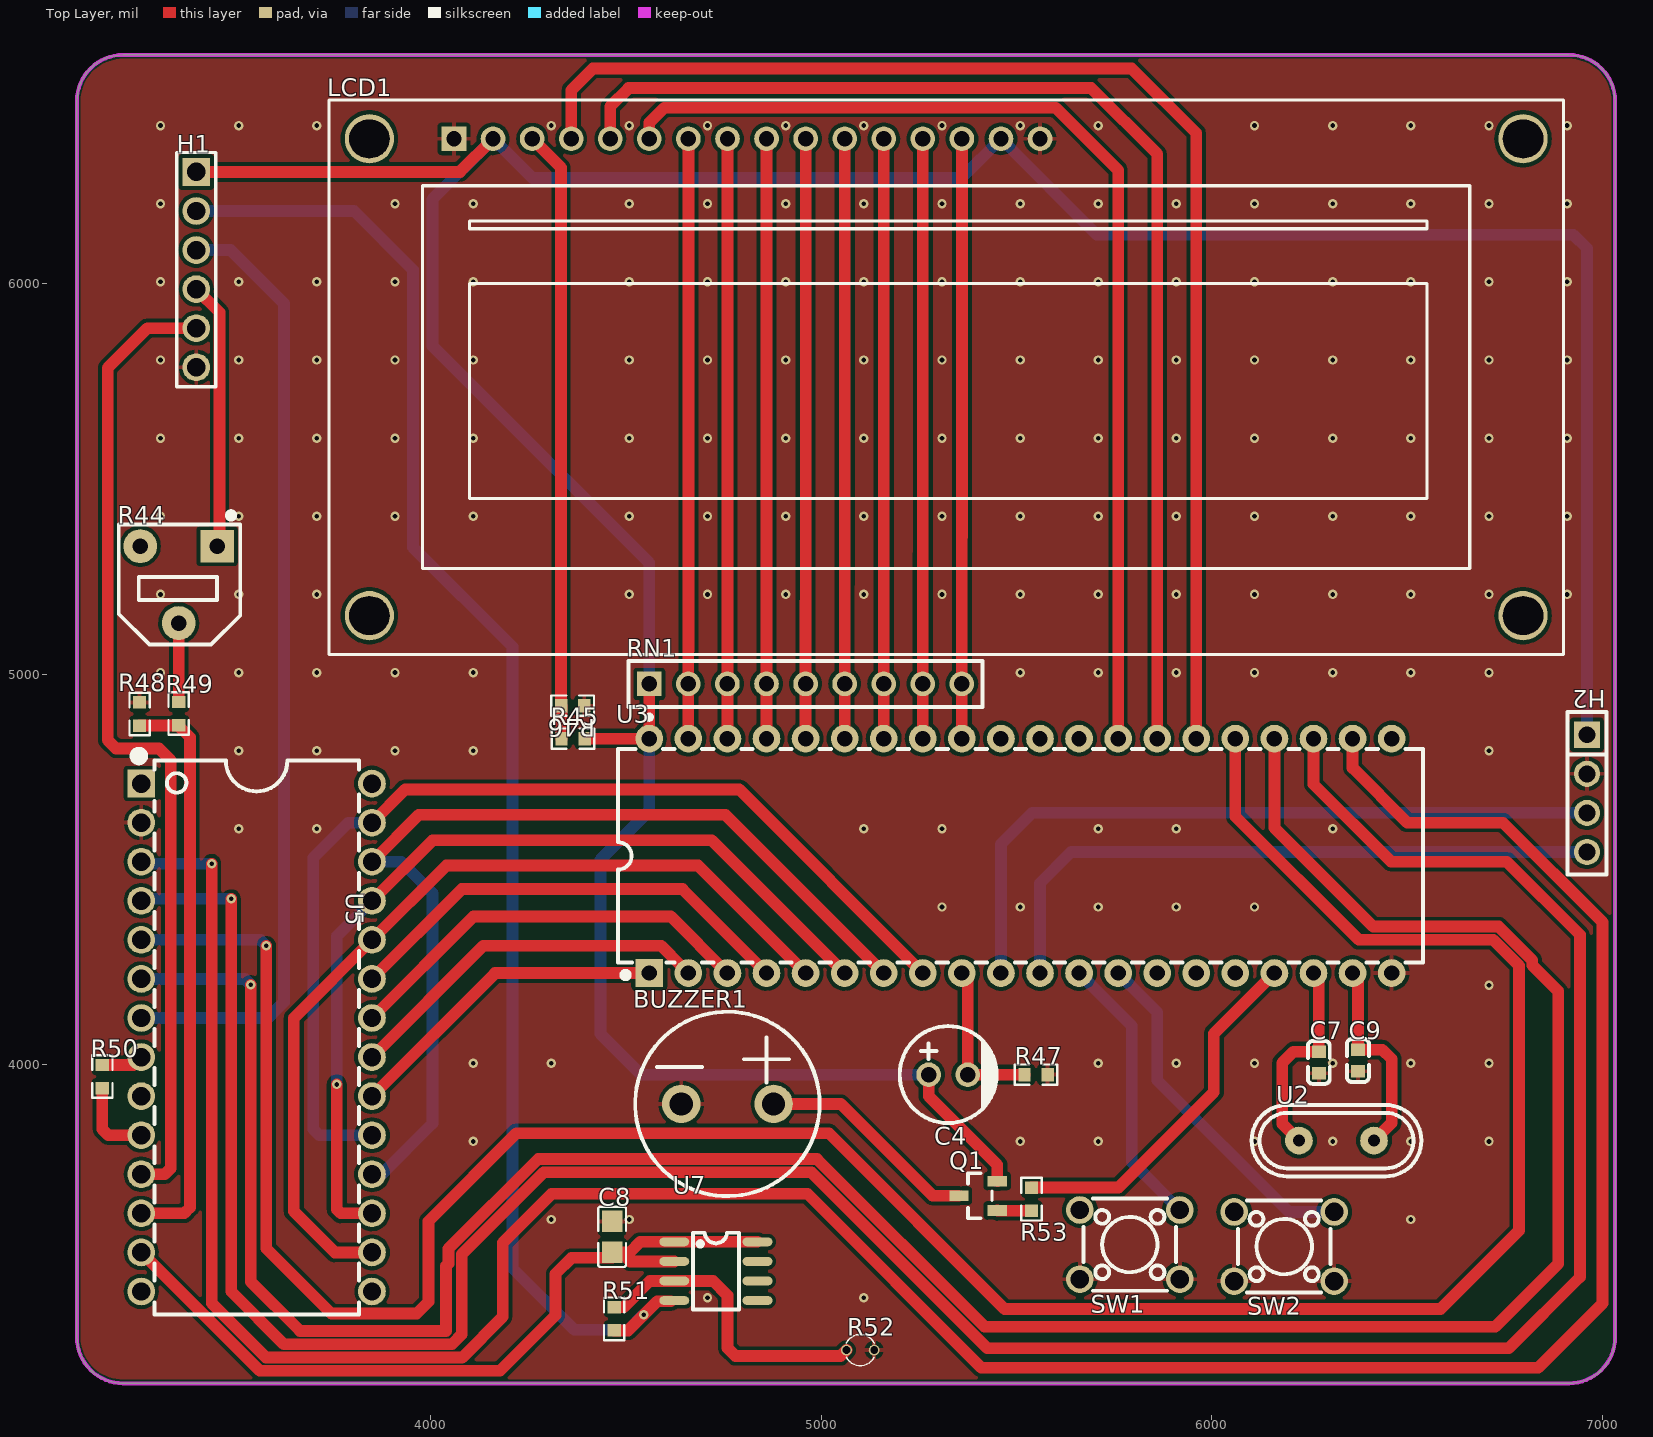
[diagram p0: Top Layer view]
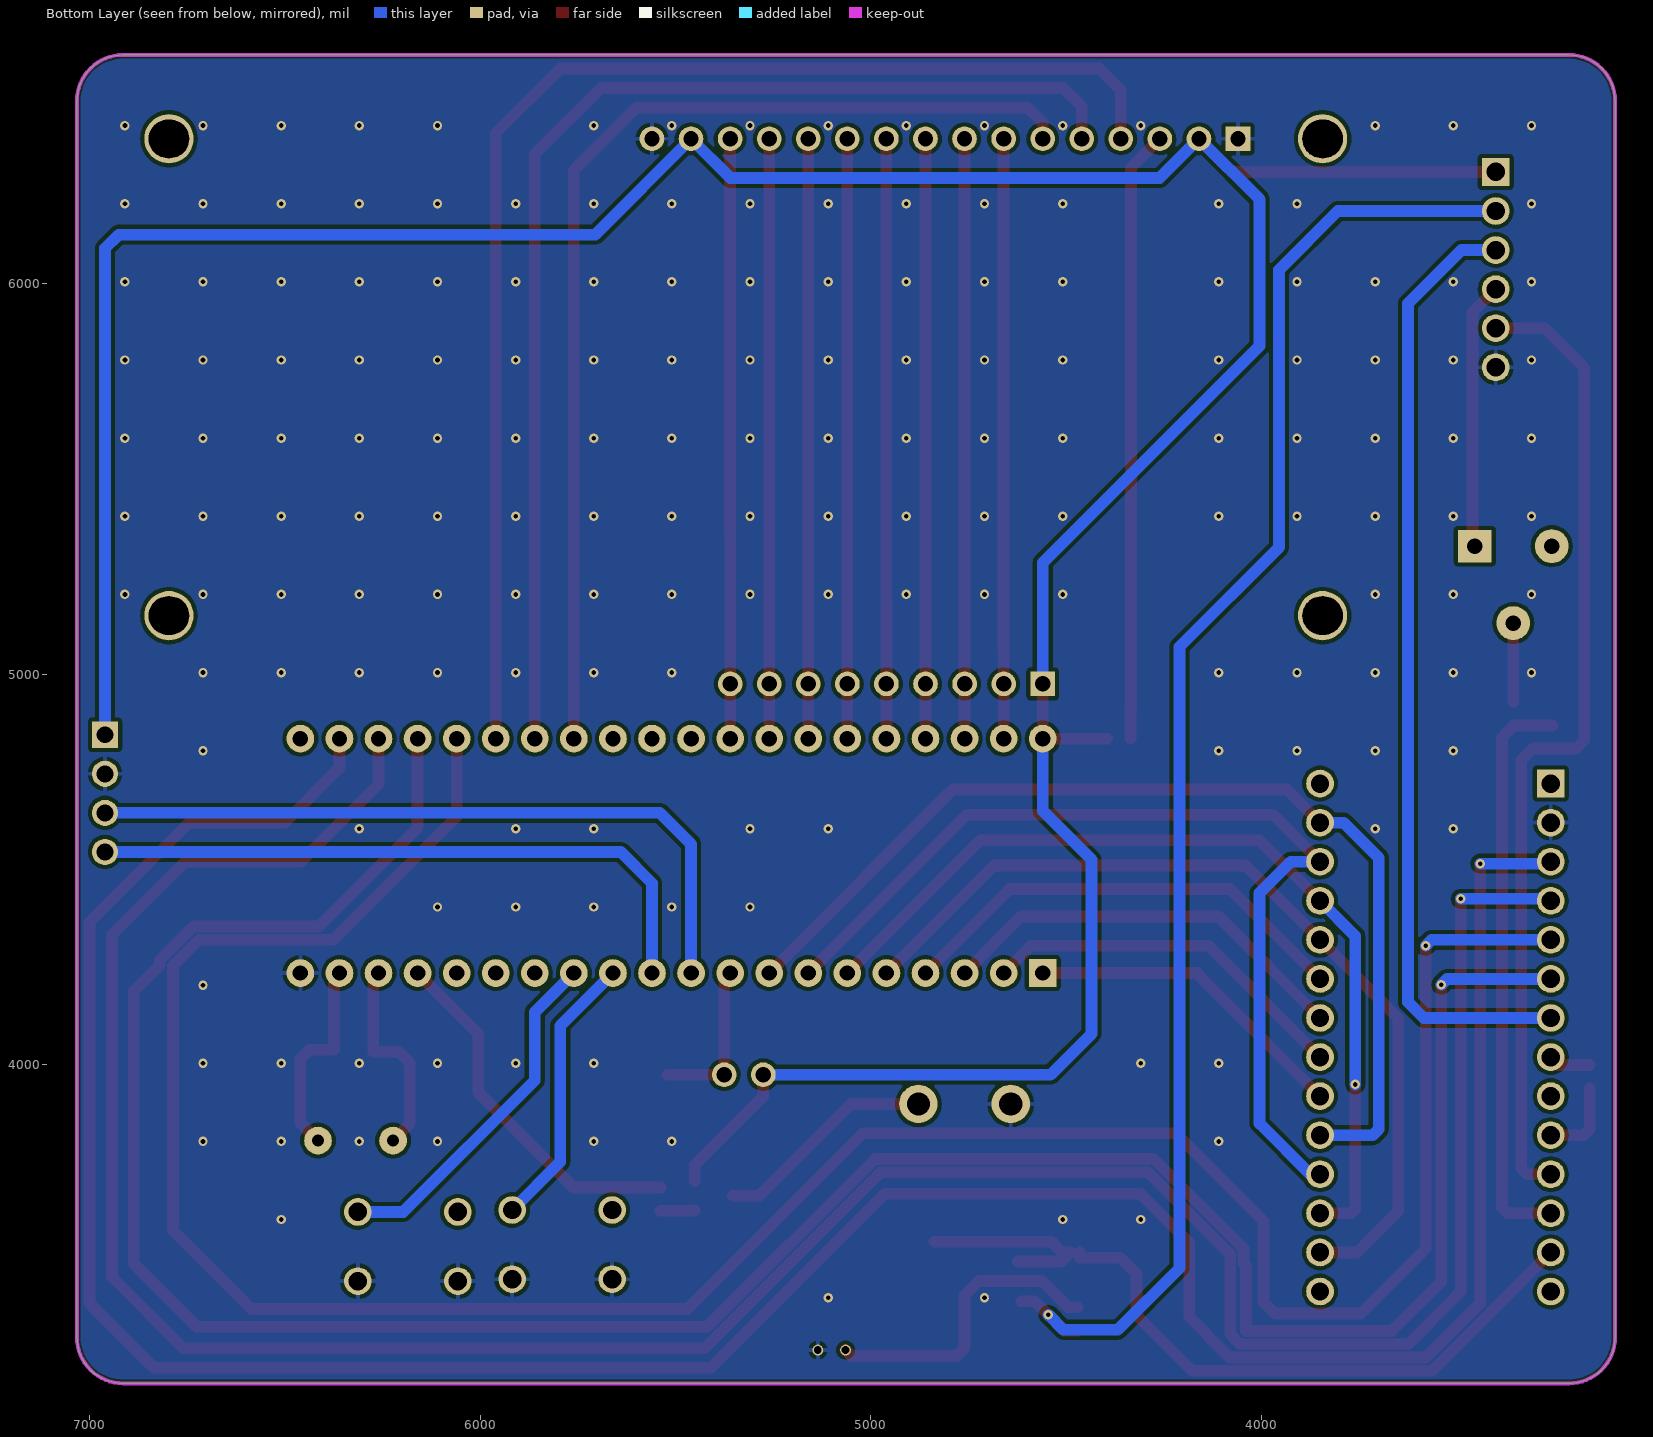
[diagram p1: Bottom Layer view, seen from below]
# Altium PCB MISC51839.pcbdoc
Units mil, origin at the board's own origin, x right, y up, seen from the top; angles counter-clockwise.
Board outline 3937.01 x 3400.14 mil, 2 copper layers (Top Layer, Bottom Layer), stack 62.206 mil thick; 26 components, 49 nets, 159 pads, 176 vias.

## Layer stack, top to bottom
Top Solder Mask Layer: solder mask 0.394, Dk 3.3
Top Layer: signal copper 1.379
Dielectric1: surface 59.449, FR4, Dk 4.5
Bottom Layer: signal copper 1.378
Bottom Solder Mask Layer: solder mask 0.394, Dk 3.3

## Board outline
3213.11,6585 ccw(c3213.11,6466.89) 3095,6466.89 3095,3302.97 ccw(c3213.11,3302.97) 3213.11,3184.86 6913.9,3184.86 ccw(c6913.9,3302.97) 7032.01,3302.97 7032.01,6466.89 ccw(c6913.9,6466.89) 6913.9,6585

## Design rules (kind name [scope] priority, off if disabled: settings)
BoardOutlineClearance copperThickness2oz_1 [All] p2 off: genericclearance=7.99 ignorepadtopadclearanceinfootprint=FALSE except(0: Arc-SplitContinuation Track-SplitContinuation SMDPad-SplitContinuation THPad-SplitContinuation Via-SplitContinuation Fill-SplitContinuation Region-SplitContinuation Poly-SplitContinuation Text-SplitContinuation Hole-SplitContinuation; 5.98: Arc-CutoutEdge Track-CutoutEdge SMDPad-CutoutEdge THPad-CutoutEdge Via-CutoutEdge Text-CutoutEdge; 6.9: Hole-OutlineEdge Hole-CutoutEdge; 10: Poly-OutlineEdge Poly-CutoutEdge; 11.81: Arc-OutlineEdge Track-OutlineEdge SMDPad-OutlineEdge THPad-OutlineEdge Via-OutlineEdge Fill-OutlineEdge Region-OutlineEdge Text-OutlineEdge Fill-CutoutEdge Region-CutoutEdge)
BoardOutlineClearance Plane_innerPlane_1 [All] p4 off: genericclearance=4.02 ignorepadtopadclearanceinfootprint=FALSE except(0: Arc-SplitContinuation Track-SplitContinuation SMDPad-SplitContinuation THPad-SplitContinuation Via-SplitContinuation Fill-SplitContinuation Region-SplitContinuation Poly-SplitContinuation Text-SplitContinuation Hole-SplitContinuation; 5.98: Arc-CutoutEdge Track-CutoutEdge SMDPad-CutoutEdge THPad-CutoutEdge Via-CutoutEdge Text-CutoutEdge; 6.9: Hole-OutlineEdge Hole-CutoutEdge; 10: Poly-OutlineEdge Poly-CutoutEdge; 11.81: Arc-OutlineEdge Track-OutlineEdge SMDPad-OutlineEdge THPad-OutlineEdge Via-OutlineEdge Fill-OutlineEdge Region-OutlineEdge Text-OutlineEdge Fill-CutoutEdge Region-CutoutEdge)
BoardOutlineClearance Copper_copperRegion_1 [All] p6 off: genericclearance=4.02 ignorepadtopadclearanceinfootprint=FALSE except(0: Arc-SplitContinuation Track-SplitContinuation SMDPad-SplitContinuation THPad-SplitContinuation Via-SplitContinuation Fill-SplitContinuation Region-SplitContinuation Poly-SplitContinuation Text-SplitContinuation Hole-SplitContinuation; 5.98: Arc-CutoutEdge Track-CutoutEdge SMDPad-CutoutEdge THPad-CutoutEdge Via-CutoutEdge Text-CutoutEdge; 6.9: Hole-OutlineEdge Hole-CutoutEdge; 10: Poly-OutlineEdge Poly-CutoutEdge; 11.81: Arc-OutlineEdge Track-OutlineEdge SMDPad-OutlineEdge THPad-OutlineEdge Via-OutlineEdge Fill-OutlineEdge Region-OutlineEdge Text-OutlineEdge Fill-CutoutEdge Region-CutoutEdge)
BoardOutlineClearance copperThickness1oz_1 [All] p8: genericclearance=4.02 ignorepadtopadclearanceinfootprint=FALSE except(0: Arc-SplitContinuation Track-SplitContinuation SMDPad-SplitContinuation THPad-SplitContinuation Via-SplitContinuation Fill-SplitContinuation Region-SplitContinuation Poly-SplitContinuation Text-SplitContinuation Hole-SplitContinuation; 5.98: Arc-CutoutEdge Track-CutoutEdge SMDPad-CutoutEdge THPad-CutoutEdge Via-CutoutEdge Text-CutoutEdge; 6.9: Hole-OutlineEdge Hole-CutoutEdge; 10: Poly-OutlineEdge Poly-CutoutEdge; 11.81: Arc-OutlineEdge Track-OutlineEdge SMDPad-OutlineEdge THPad-OutlineEdge Via-OutlineEdge Fill-OutlineEdge Region-OutlineEdge Text-OutlineEdge Fill-CutoutEdge Region-CutoutEdge)
Clearance copperThickness2oz [All] p1 off: gap=7.99 ignorepadtopadclearanceinfootprint=FALSE except(5.98: SMDPad-Track SMDPad-SMDPad THPad-Track SMDPad-THPad THPad-THPad Track-Via SMDPad-Via THPad-Via Via-Via Fill-SMDPad Region-SMDPad Fill-THPad Region-THPad Fill-Via Region-Via Fill-Fill Fill-Region Region-Region Arc-Track Arc-SMDPad Arc-THPad Arc-Via Fill-Arc Region-Arc Arc-Arc Text-Track SMDPad-Text Text-THPad Text-Via Fill-Text Region-Text Arc-Text Text-Text; 6.9: Hole-Track Hole-SMDPad Hole-THPad Hole-Via Fill-Hole Region-Hole Hole-Arc Hole-Text; 10: Poly-Track Poly-SMDPad Poly-THPad Poly-Via Poly-Fill Poly-Region Poly-Poly Poly-Arc Poly-Text Poly-Hole; 11.81: Fill-Track Region-Track)
Clearance Plane_innerPlane [All] p3 off: gap=4.02 ignorepadtopadclearanceinfootprint=FALSE except(5.98: SMDPad-Track SMDPad-SMDPad THPad-Track SMDPad-THPad THPad-THPad Track-Via SMDPad-Via THPad-Via Via-Via Fill-SMDPad Region-SMDPad Fill-THPad Region-THPad Fill-Via Region-Via Fill-Fill Fill-Region Region-Region Arc-Track Arc-SMDPad Arc-THPad Arc-Via Fill-Arc Region-Arc Arc-Arc Text-Track SMDPad-Text Text-THPad Text-Via Fill-Text Region-Text Arc-Text Text-Text; 6.9: Hole-Track Hole-SMDPad Hole-THPad Hole-Via Fill-Hole Region-Hole Hole-Arc Hole-Text; 10: Poly-Track Poly-SMDPad Poly-THPad Poly-Via Poly-Fill Poly-Region Poly-Poly Poly-Arc Poly-Text Poly-Hole; 11.81: Fill-Track Region-Track)
Clearance Copper_copperRegion [All] p5 off: gap=4.02 ignorepadtopadclearanceinfootprint=FALSE except(5.98: SMDPad-Track SMDPad-SMDPad THPad-Track SMDPad-THPad THPad-THPad Track-Via SMDPad-Via THPad-Via Via-Via Fill-SMDPad Region-SMDPad Fill-THPad Region-THPad Fill-Via Region-Via Fill-Fill Fill-Region Region-Region Arc-Track Arc-SMDPad Arc-THPad Arc-Via Fill-Arc Region-Arc Arc-Arc Text-Track SMDPad-Text Text-THPad Text-Via Fill-Text Region-Text Arc-Text Text-Text; 6.9: Hole-Track Hole-SMDPad Hole-THPad Hole-Via Fill-Hole Region-Hole Hole-Arc Hole-Text; 10: Poly-Track Poly-SMDPad Poly-THPad Poly-Via Poly-Fill Poly-Region Poly-Poly Poly-Arc Poly-Text Poly-Hole; 11.81: Fill-Track Region-Track)
Clearance copperThickness1oz [All] p7: gap=4.02 ignorepadtopadclearanceinfootprint=FALSE except(5.98: SMDPad-Track SMDPad-SMDPad THPad-Track SMDPad-THPad THPad-THPad Track-Via SMDPad-Via THPad-Via Via-Via Fill-SMDPad Region-SMDPad Fill-THPad Region-THPad Fill-Via Region-Via Fill-Fill Fill-Region Region-Region Arc-Track Arc-SMDPad Arc-THPad Arc-Via Fill-Arc Region-Arc Arc-Arc Text-Track SMDPad-Text Text-THPad Text-Via Fill-Text Region-Text Arc-Text Text-Text; 6.9: Hole-Track Hole-SMDPad Hole-THPad Hole-Via Fill-Hole Region-Hole Hole-Arc Hole-Text; 10: Poly-Track Poly-SMDPad Poly-THPad Poly-Via Poly-Fill Poly-Region Poly-Poly Poly-Arc Poly-Text Poly-Hole; 11.81: Fill-Track Region-Track)
DiffPairsRouting differentialPair [All] p1: maxlimit=6 minlimit=6 mostfreqgap=6 toplayer_minwidth=5 toplayer_prefwidth=10 toplayer_maxwidth=100 toplayer_mingap=6 toplayer_prefgap=6 toplayer_maxgap=6 bottomlayer_minwidth=5 bottomlayer_prefwidth=10 bottomlayer_maxwidth=100 bottomlayer_mingap=6 bottomlayer_prefgap=6 bottomlayer_maxgap=6 maxuncoupledlength=10
HoleToHoleClearance otherClearance [All] p1: gap=11.81 allowstackedmicrovias=TRUE
Length netLength [All] p1: minlimit=0 maxlimit=0
PasteMaskExpansion pasteMaskExpansion [All] p1: expansion=0
PlaneConnect innerPlane [All] p1: planeconnectstyle=Relief reliefexpansion=20 reliefentries=4 reliefconductorwidth=10 reliefairgap=10
PolygonConnect copperRegion [All] p1: connectstyle=Relief reliefconductorwidth=10 reliefentries=4 polygonreliefangle="90 Angle" airgapwidth=10 via.connectstyle=Relief via.reliefconductorwidth=10 via.reliefentries=4 via.polygonreliefangle="90 Angle" via.airgapwidth=10
RoutingVias viaSize [All] p1: holewidth=12.01 width=24.02 viastyle="Through Hole" minholewidth=11.81 minwidth=19.68 maxholewidth=248.03 maxwidth=393.7
SolderMaskExpansion solderMaskExpansion [IsVia] p1: expansion=-1000 istentingtop=TRUE
SolderMaskExpansion solderMaskExpansion [All] p2: expansion=2 istentingtop=FALSE
Width copperThickness2oz_2 [All] p1 off: maxlimit=100 minlimit=8 preferedwidth=10
Width copperThickness1oz_2 [All] p2: maxlimit=100 minlimit=5 preferedwidth=10

## Components (designator, comment, footprint, x,y, rotation, side; value= is the part's Value field where it differs from the comment)
BUZZER1 "buzzer" BUZ-TH_BD12.0-P6.00-D0.9-RD 4760,3900 r0 top
C4 "10uF" CAP-TH_BD6.3-P2.50-D1.0-FD 5325,3975 r0 top
C7 "22pF" C0603 6273.79,4006.21 r90 top
C8 "100nF" C0805 4465,3560 r270 top
C9 "22pF" C0603 6373.79,4011.21 r90 top
H1 "" HDR-TH_6P-P2.54-V-M-1 3400.49,6035.49 r270 top
H2 "" HDR-TH_4P-P2.54-V-F 6960,4695 r270 top
LCD1 "LMB162ADC" LCD1602 5320,5760 r0 top
Q1 "" S8550P_SOT 5400,3665 r0 top
R44 "10kΩ" RES-ADJ-SMD_RM065-V1 3355.64,5229.2 r180 top
R45 "10K" R0603 4365,4835 r0 top
R46 "1K" R0603 4363.85,4919.21 r180 top
R47 "10K" R0603 5550,3975 r180 top
R48 "100K" R0603 3255.5,4898.03 r90 top
R49 "100K" R0603 3355.64,4899.2 r90 top
R50 "50" R0603 3160,3970 r90 top
R51 "1K" R0603 4470,3350 r270 top
R52 "MF52A502F3435" RES-TH_BD2.0-P1.80-D0.3 5100,3270 r180 top
R53 "2.2K" R0603 5538.43,3656.2 r270 top
RN1 "-" RES-ARRAY-TH_9P-P2.54-D1.0 4960,4975 r0 top
SW1 "" SW-TH_4P-L6.0-W6.0-P4.50-LS6.5 5790,3540 r180 top
SW2 "" SW-TH_4P-L6.0-W6.0-P4.50-LS6.5 6185,3535 r180 top
U2 "12MHz" HC-49US_L11.0-W4.6-P4.88 6318.79,3806.21 r0 top
U3 "STC89C516RD+40I-PDIP40" DIP-40_L52.3-W13.9-P2.54-LS15.2-BL 5510,4535 r0 top
U5 "AD1674AD" CDIP-28_L35.5-W14.8-P2.54-LS15.3-BL 3555,4070 r270 top
U7 "LM358P-CN" SOIC-8_L5.0-W4.0-P1.27-LS6.0-BL 4730.48,3471.93 r270 top

## Footprints (in the part's own frame and the unit in brackets; to place one, negate y for a bottom-side part, rotate by r counter-clockwise, add the part's x,y. Pads: shape width x height; smd on the part's side, far side on the other; paste and mask are expansions set on the pad)
BUZ-TH_BD12.0-P6.00-D0.9-RD [mm]
  round 2.5 hole 1.5 paste+0 mask+0.05: 1(-3,0) 2(3,0)
  silkscreen extent -5.99,-5.99 5.99,5.99
C0603 [mm]
  rect 0.8x0.9 smd: 1(-0.7,0) 2(0.7,0)
  silkscreen extent -1.39,-0.71 1.39,0.71
C0805 [mm]
  rect 1.41x1.35 smd paste-100 mask+0.051: 1(-1,0) 2(1,0)
  silkscreen extent -1.96,-0.9 1.96,0.9
CAP-TH_BD6.3-P2.50-D1.0-FD [mm]
  round 1.6 hole 1: 1(-1.27,0) 2(1.27,0)
  silkscreen extent -3.15,-3.15 3.17,3.15
CDIP-28_L35.5-W14.8-P2.54-LS15.3-BL [mm]
  rect 1.8x1.8 hole 1.2: 1(-16.51,-7.5)
  round 1.8 hole 1.2: 2(-13.97,-7.5) 3(-11.43,-7.5) 4(-8.89,-7.5) 5(-6.35,-7.5) 6(-3.81,-7.5) 7(-1.27,-7.5) 8(1.27,-7.5) 9(3.81,-7.5) 10(6.35,-7.5) 11(8.89,-7.5) 12(11.43,-7.5) 13(13.97,-7.5) 14(16.51,-7.5) 15(16.51,7.5) 16(13.97,7.5) 17(11.43,7.5) 18(8.89,7.5) 19(6.35,7.5) 20(3.81,7.5) 21(1.27,7.5) 22(-1.27,7.5) 23(-3.81,7.5) 24(-6.35,7.5) 25(-8.89,7.5) 26(-11.43,7.5) 27(-13.97,7.5) 28(-16.51,7.5)
  silkscreen extent -18.6,-7.96 18,6.65
DIP-40_L52.3-W13.9-P2.54-LS15.2-BL [mm]
  rect 1.8x1.8 hole 1: 1(-24.13,-7.62)
  round 1.8 hole 1: 2(-21.59,-7.62) 3(-19.05,-7.62) 4(-16.51,-7.62) 5(-13.97,-7.62) 6(-11.43,-7.62) 7(-8.89,-7.62) 8(-6.35,-7.62) 9(-3.81,-7.62) 10(-1.27,-7.62) 11(1.27,-7.62) 12(3.81,-7.62) 13(6.35,-7.62) 14(8.89,-7.62) 15(11.43,-7.62) 16(13.97,-7.62) 17(16.51,-7.62) 18(19.05,-7.62) 19(21.59,-7.62) 20(24.13,-7.62) 21(24.13,7.62) 22(21.59,7.62) 23(19.05,7.62) 24(16.51,7.62) 25(13.97,7.62) 26(11.43,7.62) 27(8.89,7.62) 28(6.35,7.62) 29(3.81,7.62) 30(1.27,7.62) 31(-1.27,7.62) 32(-3.81,7.62) 33(-6.35,7.62) 34(-8.89,7.62) 35(-11.43,7.62) 36(-13.97,7.62) 37(-16.51,7.62) 38(-19.05,7.62) 39(-21.59,7.62) 40(-24.13,7.62)
  silkscreen extent -26.16,-7.95 26.16,6.93
HC-49US_L11.0-W4.6-P4.88 [mm]
  round 1.8 hole 0.8: 1(-2.44,0) 2(2.44,0)
  silkscreen extent -5.51,-2.32 5.51,2.32
HDR-TH_4P-P2.54-V-F [mm]
  rect 1.7x1.7 hole 1.1: 1(-3.81,0)
  round 1.7 hole 1.1: 2(-1.27,0) 3(1.27,0) 4(3.81,0)
  silkscreen extent -5.29,-1.27 5.29,1.27
HDR-TH_6P-P2.54-V-M-1 [mm]
  rect 1.8x1.8 hole 1.2: 1(-6.35,0)
  round 1.8 hole 1.2: 2(-3.81,0) 3(-1.27,0) 4(1.27,0) 5(3.81,0) 6(6.35,0)
  silkscreen extent -7.62,-1.27 7.62,1.27
LCD1602 [mm]
  round 3.2 hole 2.5 slot 2.625 at 0 deg: 0(-37.5,-15.5) 0(-37.5,15.5) 0(37.5,-15.5) 0(37.5,15.5)
  rect 1.6x1.6 hole 1: 1(-32,15.5)
  round 1.6 hole 1: 2(-29.46,15.5) 3(-26.92,15.5) 4(-24.38,15.5) 5(-21.84,15.5) 6(-19.3,15.5) 7(-16.76,15.5) 8(-14.22,15.5) 9(-11.68,15.5) 10(-9.14,15.5) 11(-6.6,15.5) 12(-4.06,15.5) 13(-1.52,15.5) 14(1.02,15.5) 15(3.56,15.5) 16(6.1,15.5)
  silkscreen extent -40.13,-18.03 40.13,18.03
R0603 [mil]
  rect 31.75x34.02 smd paste-3937.01 mask+2: 1(-29.66,0) 2(29.66,0)
  silkscreen extent -55,-26 55,26
RES-ADJ-SMD_RM065-V1 [mm]
  rect 2.2x2.1 hole 1 paste+0 mask+0.05: 1(-2.5,-2.5)
  round 2.2 hole 1 paste+0 mask+0.05: 2(0,2.5) 3(2.5,-2.5)
  silkscreen extent -4,-4.7 3.9,3.9
RES-ARRAY-TH_9P-P2.54-D1.0 [mm]
  rect 1.6x1.6 hole 1: 1(-10.16,0)
  round 1.6 hole 1: 2(-7.62,0) 3(-5.08,0) 4(-2.54,0) 5(0,0) 6(2.54,0) 7(5.08,0) 8(7.62,0) 9(10.16,0)
  silkscreen extent -11.5,-2.31 11.5,1.5
RES-TH_BD2.0-P1.80-D0.3 [mm]
  round 0.7 hole 0.5 paste+0 mask+0.05: 1(-0.9,0) 2(0.9,0)
  silkscreen extent -0.91,-1.01 0.91,1.01
S8550P_SOT [mil]
  rect 49.2x27.6 smd paste+0 mask+2: 1(50.84,-37.4) 2(50.84,37.4) 3(-47.56,0)
  silkscreen extent -24,-58 37,58
SOIC-8_L5.0-W4.0-P1.27-LS6.0-BL [mil]
  oval 22.38x76.78 smd: 1(-75,-106.5) 2(-25,-106.5) 3(25,-106.5) 4(75,-106.5) 5(75,106.5) 6(25,106.5) 7(-25,106.5) 8(-75,106.5)
  silkscreen extent -98,-59 98,59
SW-TH_4P-L6.0-W6.0-P4.50-LS6.5 [mm]
  round 1.8 hole 1.2: 1(-3.25,2.25) 2(3.25,2.25) 3(-3.25,-2.25) 4(3.25,-2.25)
  silkscreen extent -3,-3 3,3

## Via types
v1: diameter 24.02, hole 12, Top Layer to Bottom Layer, 176 vias

## Nets (pads, with @x,y where several pads share a name; then routed paths per layer and width w, separated by ;. In a path a pad name is that pad's centre, name@x,y a point inside that pad or via, vN(x,y) a via of type N, cw(c..) or ccw(c..) an arc to the next point about the centre after c; other vN are vias at no path point)
$1N1586: LCD1.14 RN1.9 U3.32 | length 1535.3
  Top Layer w30: U3.32 RN1.9 5360,5351.13 5360.16,5351.29 LCD1.14
$1N1590: LCD1.7 RN1.2 U3.39 | length 1535.3
  Top Layer w30: U3.39 RN1.2 4660,5061.18 4660.16,5061.34 LCD1.7
$1N1591: LCD1.8 RN1.3 U3.38 | length 1535.3
  Top Layer w30: U3.38 RN1.3 4760,5102.6 4760.16,5102.76 LCD1.8
$1N1592: LCD1.9 RN1.4 U3.37 | length 1535.3
  Top Layer w30: U3.37 RN1.4 4860,5144.02 4860.16,5144.18 LCD1.9
$1N1593: LCD1.10 RN1.5 U3.36 | length 1535.3
  Top Layer w30: U3.36 RN1.5 4960,5185.44 4960.16,5185.6 LCD1.10
$1N1594: LCD1.11 RN1.6 U3.35 | length 1535.3
  Top Layer w30: U3.35 RN1.6 5060,5226.86 5060.16,5227.02 LCD1.11
$1N1595: LCD1.12 RN1.7 U3.34 | length 1535.3
  Top Layer w30: U3.34 RN1.7 5160,5268.28 5160.16,5268.44 LCD1.12
$1N1596: LCD1.13 RN1.8 U3.33 | length 1535.3
  Top Layer w30: U3.33 RN1.8 5260,5309.7 5260.16,5309.86 LCD1.13
$1N1605: LCD1.3 R45.1 R46.2 | length 1566.4
  Top Layer w30: LCD1.3 4334.19,6296.21 R46.2 4335.34,4918.06 R45.1
$1N1611: C7.2 U2.1 U3.18 | length 529.1
  Top Layer w30: U2.1 6180,3848.94 6180,4005 6208.77,4033.77 C7.2 6273.79,4221.21 U3.18
$1N1612: C9.2 U2.2 U3.19 | length 525.5
  Top Layer w30: U3.19 6373.79,4221.21 C9.2 6436.23,4038.77 6460,4015 6460,3851.36 U2.2@6414.85,3806.21
$1N22801: C4.2 R47.2 U3.9 | length 411.6
  Top Layer w30: U3.9 5375,4220 C4.2 R47.2
$1N22819: U3.1 U5.20 | length 840.2
  Top Layer w30: U5.20 4165.27,4235 U3.1
$1N22823: U3.2 U5.21 | length 957.1
  Top Layer w30: U5.21 4135.27,4305 4590.54,4305 4616.42,4279.12 4616.42,4278.58 U3.2
$1N22827: U3.8 U5.19 U5.27 | length 2678.6
  Top Layer w30: U5.27 3935.27,4705 4790,4705 U3.8
  Bottom Layer w30: U5.19 3715,3820 3700,3835 3700,4530 3790,4620 U5.27
$1N22836: U3.7 U5.18 U5.26 | length 2513.6
  Top Layer w30: U5.26 3970.27,4640 4755,4640 U3.7
  Bottom Layer w30: U5.18 3875,3720 4005,3850 4005,4440 3925,4520 U5.26
$1N22841: U3.6 U5.17 U5.25 | length 2336.6
  Top Layer w30: v1(3760,3950) 3760,3630 3770,3620 U5.17 ; U5.25 4005.27,4575 4720,4575 U3.6
  Bottom Layer w30: v1(3760,3950) 3760,4329.73 U5.25
$1N22846: U3.5 U5.16 U5.24 | length 2324.1
  Top Layer w30: U5.16 3755,3520 3650,3625 3650,4119.73 U5.24 4040.27,4510 4685,4510 U3.5
$1N22851: U3.4 U5.23 | length 1194.1
  Top Layer w30: U5.23 4080.27,4450 4645,4450 U3.4
$1N22856: U3.3 U5.22 | length 1077.5
  Top Layer w30: U5.22 4110.27,4380 4615,4380 U3.3
$1N23012: R50.2 U5.8 | length 108.2
  Top Layer w30: R50.2 3239.39,3999.66 U5.8
$1N23018: R50.1 U5.10 | length 211.3
  Top Layer w30: R50.1 3160,3835 3175,3820 U5.10
$1N23025: R48.1 R49.1 U5.12 | length 1477.4
  Top Layer w30: R48.1 R49.1@3354.47,4868.37 ; U5.12 3369.47,3620 3384.47,3635 3384.47,4838.37 R49.1@3354.47,4868.37 ; R49.1 R49.1@3354.47,4868.37
$1N23497: C8.2 U5.13 U7.1 U7.2 U7.8 | length 2033.2
  Top Layer w30: U5.13 3562.92,3216.81 4178,3216.81 4320,3358.81 4320,3465 4361.08,3506.08 4465,3506.08 C8.2 ; U7.2 4511.64,3496.93 4487.95,3520.63 4510.63,3520.63 4536.93,3546.93 U7.1 U7.8
$1N23895: R51.1 R52.2 U7.3 | length 786.9
  Top Layer w30: R51.1 4494.66,3379.66 4561.93,3446.93 U7.3 4723.07,3446.93 4760,3410 4760,3275.52 4780.52,3255 5049.56,3255 R52.2
$1N24757: R44.2 R49.2 | length 201.9
  Top Layer w30: R49.2 R44.2
$1N26077: H2.3 U3.10 | length 1863.1
  Bottom Layer w30: U3.10 5460,4565 5540,4645 H2.3
$1N26083: H2.4 U3.11 | length 1663.1
  Bottom Layer w30: U3.11 5560,4465 5640,4545 H2.4
$1N26653: R53.1 U3.17 | length 936.9
  Top Layer w30: R53.1 5760.86,3685.86 6005,3930 6005,4080 U3.17
$1N27309: Q1.1 R53.2 | length 88
  Top Layer w30: Q1.1 5451.89,3626.55 R53.2
$1N27395: BUZZER1.2 Q1.3 | length 571.7
  Top Layer w30: BUZZER1.2 5050,3900 5285,3665 Q1.3
$1N27471: SW1.3 U3.12 | length 713.3
  Bottom Layer w30: U3.12 5795,4100 5795,3751.53 SW1.3
$1N27486: SW2.3 U3.13 | length 908.7
  Bottom Layer w30: U3.13 5860,4135 5860,3960 6196.42,3623.58 SW2.3
+6V: H1.2 R51.2 U7.4 | length 3869.6
  Top Layer w30: R51.2 4505.92,3320.34 v1(4546.11,3360.54) 4580.58,3395 U7.4@4615,3395
  Bottom Layer w30: H1.2 3804.51,6185.49 3955,6035 3955,5325 4210,5070 4210,3480 4368.07,3321.93 4506.93,3321.93 v1@4545,3360
+12V: H1.4 R44.1 | length 685
  Top Layer w30: H1.4 3460,5925.98 3460,5333.56 R44.1
+16V: H1.3 U5.7 | length 2451.8
  Bottom Layer w30: U5.7 3585,4120 3625,4160 3625,5948.84 3488.35,6085.49 H1.3
-12V: R44.3
-15V: H1.5 U5.11 | length 2530.3
  Top Layer w30: U5.11 3320,3720 3335,3735 3335,4780 3305,4810 3195,4810 3173.79,4831.21 3173.79,5783.79 3275.49,5885.49 H1.5
AD: U3.23 U5.4 | length 7143.6
  Top Layer w30: v1(3490,4425) 3490,3420 3625,3285 4055,3285 4080,3310 4080,3515 4290,3725 4975,3725 5425,3275 6760,3275 6942.09,3457.09 6942.09,4332.91 6755,4520 6458.58,4520 6260,4718.58 U3.23
  Bottom Layer w30: U5.4 3264.73,4425 v1(3490,4425)
CE: U3.24 U5.6 | length 6823.8
  Top Layer w30: v1(3540,4205) 3540,3445 3665.98,3319.02 4040,3319.02 4040,3485 4045.98,3490.98 4045.98,3529.09 4275.91,3759.02 4989.09,3759.02 5418.11,3330 6725,3330 6886.21,3491.21 6886.21,4188.79 6820.23,4254.77 6820.23,4267.88 6734.09,4354.02 6413.14,4354.02 6160,4607.16 U3.24
  Bottom Layer w30: U5.6 3525,4220 v1(3540,4205)
CS: U3.22 U5.3 | length 7316.2
  Top Layer w30: v1(3440,4515) 3440,3390 3579.17,3250.83 4080.83,3250.83 4185,3355 4185,3545 4310,3670 4965,3670 5410,3225 6835,3225 7000,3390 7000,4365 6745,4620 6500,4620 6360,4760 U3.22
  Bottom Layer w30: U5.3 3264.73,4515 v1(3440,4515)
EN: LCD1.6 U3.28 | length 2778.5
  Top Layer w30: LCD1.6 4560.16,6411.74 4598.42,6450 5600,6450 5760,6290 U3.28
GND: BUZZER1.1 C7.1 C8.1 C9.1 H1.6 H2.2 LCD1.1 LCD1.16 R46.1 R47.1 R48.2 R52.1 SW1.1 SW1.2 SW2.1 SW2.2 U3.20 U5.2
  other v1: 4709.1,3404.1 5109.1,3404.1 4309.1,3604.1 4509.1,3604.1 6509.1,3604.1 4109.1,3804.1 5509.1,3804.1 5709.1,3804.1 6109.1,3804.1 6309.1,3804.1 6509.1,3804.1 6709.1,3804.1 4109.1,4004.1 4309.1,4004.1 5709.1,4004.1 5909.1,4004.1 6109.1,4004.1 6309.1,4004.1 6509.1,4004.1 6709.1,4004.1 6709.1,4204.1 5309.1,4404.1 5509.1,4404.1 5709.1,4404.1 5909.1,4404.1 6109.1,4404.1 3509.1,4604.1 3709.1,4604.1 5109.1,4604.1 5309.1,4604.1 5709.1,4604.1 5909.1,4604.1 6309.1,4604.1 3509.1,4804.1 3709.1,4804.1 3909.1,4804.1 4109.1,4804.1 6709.1,4804.1 3309.1,5004.1 3509.1,5004.1 3709.1,5004.1 3909.1,5004.1 4109.1,5004.1 5509.1,5004.1 5709.1,5004.1 5909.1,5004.1 6109.1,5004.1 6309.1,5004.1 6509.1,5004.1 6709.1,5004.1 3309.1,5204.1 3509.1,5204.1 3709.1,5204.1 4509.1,5204.1 4709.1,5204.1 4909.1,5204.1 5109.1,5204.1 5309.1,5204.1 5509.1,5204.1 5709.1,5204.1 5909.1,5204.1 6109.1,5204.1 6309.1,5204.1 6509.1,5204.1 6709.1,5204.1 6909.1,5204.1 3309.1,5404.1 3509.1,5404.1 3709.1,5404.1 3909.1,5404.1 4109.1,5404.1 4509.1,5404.1 4709.1,5404.1 4909.1,5404.1 5109.1,5404.1 5309.1,5404.1 5509.1,5404.1 5709.1,5404.1 5909.1,5404.1 6109.1,5404.1 6309.1,5404.1 6509.1,5404.1 6709.1,5404.1 6909.1,5404.1 3309.1,5604.1 3509.1,5604.1 3709.1,5604.1 3909.1,5604.1 4109.1,5604.1 4509.1,5604.1 4709.1,5604.1 4909.1,5604.1 5109.1,5604.1 5309.1,5604.1 5509.1,5604.1 5709.1,5604.1 5909.1,5604.1 6109.1,5604.1 6309.1,5604.1 6509.1,5604.1 6709.1,5604.1 6909.1,5604.1 3309.1,5804.1 3509.1,5804.1 3709.1,5804.1 3909.1,5804.1 4109.1,5804.1 4509.1,5804.1 4709.1,5804.1 4909.1,5804.1 5109.1,5804.1 5309.1,5804.1 5509.1,5804.1 5709.1,5804.1 5909.1,5804.1 6109.1,5804.1 6309.1,5804.1 6509.1,5804.1 6709.1,5804.1 6909.1,5804.1 3309.1,6004.1 3509.1,6004.1 3709.1,6004.1 3909.1,6004.1 4109.1,6004.1 4509.1,6004.1 4709.1,6004.1 4909.1,6004.1 5109.1,6004.1 5309.1,6004.1 5509.1,6004.1 5709.1,6004.1 5909.1,6004.1 6109.1,6004.1 6309.1,6004.1 6509.1,6004.1 6709.1,6004.1 6909.1,6004.1 3309.1,6204.1 3909.1,6204.1 4109.1,6204.1 4509.1,6204.1 4709.1,6204.1 4909.1,6204.1 5109.1,6204.1 5309.1,6204.1 5509.1,6204.1 5709.1,6204.1 5909.1,6204.1 6109.1,6204.1 6309.1,6204.1 6509.1,6204.1 6709.1,6204.1 6909.1,6204.1 3309.1,6404.1 3509.1,6404.1 3709.1,6404.1 4309.1,6404.1 4509.1,6404.1 4709.1,6404.1 4909.1,6404.1 5109.1,6404.1 5309.1,6404.1 5509.1,6404.1 5709.1,6404.1 6109.1,6404.1 6309.1,6404.1 6509.1,6404.1 6709.1,6404.1 6909.1,6404.1
RC: U3.25 U5.5 | length 6719.7
  Top Layer w30: v1(3580,4305) 3580,3530 3746.42,3363.58 3965,3363.58 3995,3393.58 3995,3600 4220,3825 5020,3825 5470,3375 6585,3375 6786.21,3576.21 6786.21,4253.79 6720,4320 6375.74,4320 6060,4635.74 U3.25
  Bottom Layer w30: U5.5 3565,4320 v1(3580,4305)
RS: LCD1.4 U3.26 | length 3365.5
  Top Layer w30: LCD1.4 4360.16,6494.58 4415.58,6550 5795,6550 5960,6385 U3.26
RW: LCD1.5 U3.27 | length 3068.4
  Top Layer w30: LCD1.5 4460.16,6453.16 4507,6500 5691.42,6500 5860,6331.42 U3.27
STS: U5.28
SYS: U3.21
VCC: C4.1 H1.1 H2.1 LCD1.2 LCD1.15 Q1.2 R45.2 RN1.1 U3.40 | length 9069.2
  Top Layer w30: H1.1 4075.41,6285.49 LCD1.2 ; R45.2 U3.40 RN1.1 ; C4.1 5275,3920 5450.84,3744.16 Q1.2
  Bottom Layer w30: U3.40 4560,4650 4435,4525 4435,4080 4540,3975 C4.1 ; RN1.1 4560,5285 4005,5840 4005,6215.08 LCD1.2 4260.4,6270 5359.92,6270 LCD1.15 5705.4,6125 6925,6125 6960,6090 H2.1
pads on no net: LCD1.0 SW1.4 SW2.4 U3.14 U3.15 U3.16 U3.29 U3.30 U3.31 U5.1 U5.9 U5.14 U5.15 U7.5 U7.6 U7.7

## Polygon pours and split planes (outlines as drawn)
GND on Top Layer (solid, remove dead copper, pour order 0): 3000,6705 3000,3000 7365,3000 7365,6705
GND on Bottom Layer (solid, remove dead copper, pour order 2): 3035,6705 3035,3100 7420,3100 7420,6705

## Keep-outs
Board Outline Layer:
  the board outline again, w10